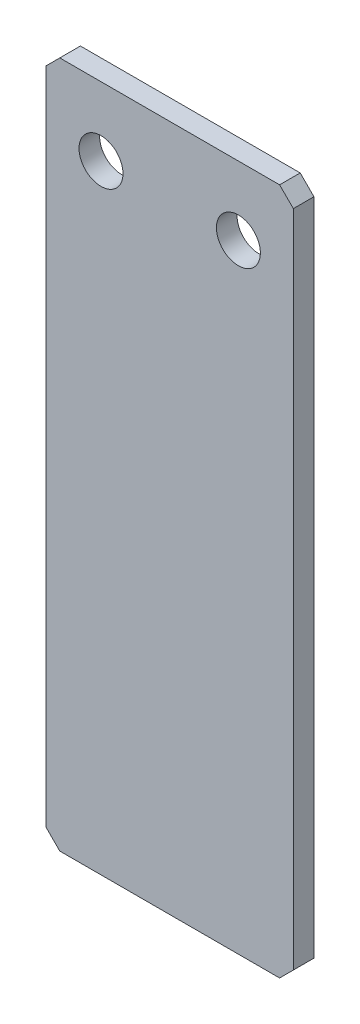
SolidWorks part; units mm, degrees
ref_plane "Front Plane" through (0, 0, 0) normal (0, 0, 1) x (1, 0, 0)
ref_plane "Top Plane" through (0, 0, 0) normal (0, 1, 0) x (1, 0, 0)
ref_plane "Right Plane" through (0, 0, 0) normal (1, 0, 0) x (0, 0, -1)
sketch "Sketch1" plane through (0, 0, 0) normal (0, 0, 1) x (1, 0, 0)
  line L1 (-9, 25) -> (9, 25)
  line L2 (-9, 25) -> (-9, -25)
  line L3 (-9, -25) -> (9, -25)
  line L4 (9, 25) -> (9, -25)
  line L5 (-9, 25) -> (9, -25) construction
  line L6 (-9, -25) -> (9, 25) construction
  point P0 (0, 0)
  dimension "D1" = 18
  dimension "D2" = 50
extrude "Boss-Extrude1" add sketch "Sketch1" along normal blind 1.5
hole_wizard "Ø3.2 (3.2) Diameter Hole1" positions "Sketch3" profile "Sketch2" hole size "Ø3.2" standard "GB"
sketch "Sketch3" plane through (0, 0, 1.5) normal (0, 0, 1) x (1, 0, 0)
  line L0 (0, 0) -> (0, 31.9643) construction
  line L2 (9, 25) -> (-9, 25) construction
  point P0 (-5, 20)
  point P1 (5, 20)
  dimension "D1" = 10
  dimension "D2" = 5
sketch "Sketch2" plane through (-5, 20, 1.5) normal (1, 0, 0) x (0, -1, 0)
  line L0 (0, 0) -> (0, 12.9614)
  line L1 (0, 12.9614) -> (1.6, 12)
  line L2 (1.6, 12) -> (1.6, 0)
  line L5 (1.6, 0) -> (0, 0)
  line L10 (0, 12.9614) -> (-1.6, 12) construction
  line L11 (0, -6.35) -> (0, 107.95) construction
  dimension "孔直径" = 3.2
  dimension "孔深度" = 12
  dimension "导头角度" = 118
chamfer "Chamfer1" distance 1 angle 45 4 edges at (-9, 25, 0.75) (9, 25, 0.75) (9, -25, 0.75) (-9, -25, 0.75)
